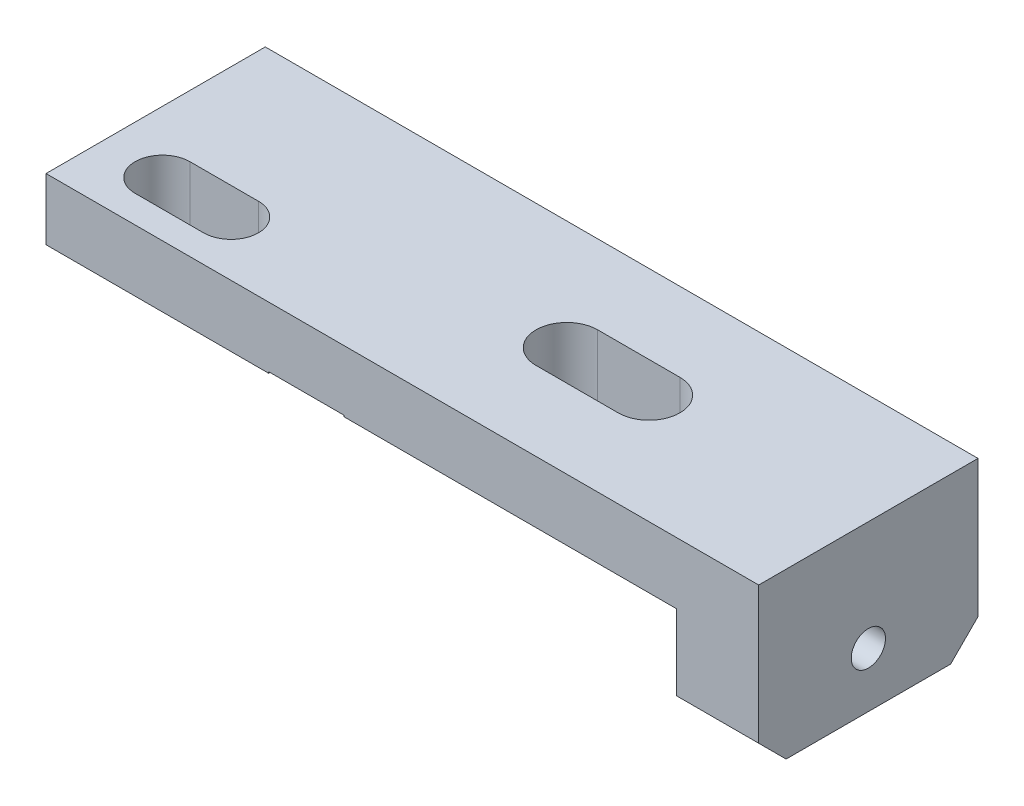
SolidWorks part; units mm, degrees
ref_plane "Front Plane" through (0, 0, 0) normal (0, 0, 1) x (1, 0, 0)
ref_plane "Top Plane" through (0, 0, 0) normal (0, 1, 0) x (1, 0, 0)
ref_plane "Right Plane" through (0, 0, 0) normal (1, 0, 0) x (0, 0, -1)
sketch "Sketch1" plane through (0, 0, 0) normal (0, 1, 0) x (1, 0, 0)
  line L1 (-23, 8) -> (23, 8)
  line L2 (-23, 8) -> (-23, -8)
  line L3 (-23, -8) -> (23, -8)
  line L4 (23, 8) -> (23, -8)
  line L5 (-23, 8) -> (23, -8) construction
  line L6 (-23, -8) -> (23, 8) construction
  point P0 (0, 0)
  dimension "D1" = 16
  dimension "D2" = 46
extrude "Boss-Extrude1" add sketch "Sketch1" along normal blind 4.5
sketch "Sketch2" plane through (23, 0, 0) normal (1, 0, 0) x (0, 0, -1)
  line L0 (8, 4.5) -> (8, 0) construction
  line L1 (-8, 4.5) -> (8, 4.5)
  line L2 (-8, 4.5) -> (-8, -7.5)
  line L3 (-8, -7.5) -> (8, -7.5)
  line L4 (8, 4.5) -> (8, -7.5)
  dimension "D1" = 12
extrude "Boss-Extrude2" add sketch "Sketch2" along normal blind 6
sketch "Sketch3" plane through (29, 0, 0) normal (1, 0, 0) x (0, 0, -1)
  line L0 (0, 0) -> (0, -50000) construction
  line L1 (-8, -7.5) -> (8, -7.5) construction
  circle A0 centre (0, -3.5) radius 1
  dimension "D1" = 2
  dimension "D2" = 4
extrude "Cut-Extrude1" cut sketch "Sketch3" against normal blind 10
hole_wizard "M3 Tapped Hole1" positions "3DSketch1" profile "Sketch4" tap size "M3" standard "Gb"
sketch3d "3DSketch1"
  line L0 (23, -3.5, 0) -> (29, -3.5, 0) construction
  point P0 (29, -3.5, 0)
sketch "Sketch4" plane through (29, -3.5, 0) normal (0, 1, 0) x (0, 0, -1)
  line L0 (0, 0) -> (0, 8.2511)
  line L1 (0, 8.2511) -> (1.25, 7.5)
  line L2 (1.25, 7.5) -> (1.25, 0)
  line L5 (1.25, 0) -> (0, 0)
  line L10 (0, 8.2511) -> (-1.25, 7.5) construction
  line L11 (0, -6.35) -> (0, 107.95) construction
  dimension "螺纹孔钻头直径" = 2.5
  dimension "螺纹孔钻头深度" = 7.5
  dimension "导头角度" = 118
cosmetic thread "Cosmetic Thread1" parameters "D1"=6, "D2"=3
chamfer "Chamfer1" distance 2 angle 45 2 edges at (26, -7.5, -8) (26, -7.5, 8)
ref_plane "Plane1" through (-5.5, 0, 0) normal (-1, 0, 0) x (0, 0, 1)
sketch "Sketch5" plane through (-5.5, 0, 0) normal (-1, 0, 0) x (0, 0, 1)
  line L0 (8, 0) -> (-8, 0) construction
  line L1 (-1.4, 0) -> (-15.0048, 0)
  line L2 (-1.4, 0) -> (-15.0048, 2.8918)
  line L3 (-15.0048, 2.8918) -> (-15.0048, 0)
  line L4 (-8, -5.5) -> (-8, 4.5) construction
  dimension "D1" = 12
  dimension "D2" = 6.6
extrude "Cut-Extrude2" cut sketch "Sketch5" against normal mid plane 15
ref_plane "Plane2" through (-4, 0, 0) normal (-1, 0, 0) x (0, 0, 1)
sketch "Sketch6" plane through (-4, 0, 0) normal (-1, 0, 0) x (0, 0, 1)
  line L7 (-1.3792, 0.0978) -> (-7.9792, 1.5007)
  line L8 (-1.3895, 0.1) -> (-8, 1.5051)
  line L9 (-8, -0.5) -> (-8, 1.5051)
  line L10 (8, 0.1) -> (-8, 0.1)
  line L11 (8, 0.1) -> (-1.3895, 0.1)
  line L12 (-8, -5.5) -> (-8, 4.5) construction
  line L13 (-8, -0.5) -> (8, -0.5)
  line L14 (8, 0.1) -> (8, -0.5)
  line L16 (8, 4.5) -> (8, -5.5) construction
  dimension "D1" = 0.1
  dimension "D2" = 0.1
extrude "Cut-Extrude3" cut sketch "Sketch6" against normal mid plane 5.5
fillet "Fillet1" radius 3 1 edges at (-4, 1.5051, -8)
fillet "Fillet2" radius 2 1 edges at (-4, 0.1, -1.3895)
sketch "Sketch7" plane through (0, 4.5, 0) normal (0, 1, 0) x (1, 0, 0)
  line L0 (-18.5, -4) -> (-13.5, -4) construction
  line L1 (-18.5, -2) -> (-13.5, -2)
  line L2 (-18.5, -6) -> (-13.5, -6)
  line L3 (29, 8) -> (-23, 8) construction
  line L4 (-23, 8) -> (-23, -8) construction
  arc A0 (-18.5, -2) -> (-18.5, -6) centre (-18.5, -4) ccw
  arc A1 (-13.5, -6) -> (-13.5, -2) centre (-13.5, -4) ccw
  point P2 (-16, -4)
  dimension "D1" = 4
  dimension "D2" = 12
  dimension "D3" = 7
  dimension "D4" = 5
extrude "Cut-Extrude4" cut sketch "Sketch7" against normal blind 15
sketch "Sketch8" plane through (0, 4.5, 0) normal (0, 1, 0) x (1, 0, 0)
  line L0 (-23, 0) -> (49977, 0) construction
  line L1 (-23, 8) -> (-23, -8) construction
  line L2 (7, 0) -> (13, 0) construction
  line L3 (7, 2.25) -> (13, 2.25)
  line L4 (7, -2.25) -> (13, -2.25)
  line L5 (29, 8) -> (29, -8) construction
  arc A0 (7, 2.25) -> (7, -2.25) centre (7, 0) ccw
  arc A1 (13, -2.25) -> (13, 2.25) centre (13, 0) ccw
  point P4 (-23, 0)
  point P7 (10, 0)
  dimension "D1" = 4.5
  dimension "D2" = 6
  dimension "D3" = 19
extrude "Cut-Extrude5" cut sketch "Sketch8" against normal blind 15
chamfer "Chamfer2" distance 0.5 angle 45 2 edges at (-6.75, 2.6687, -8) (-1.25, 2.6687, -8)
